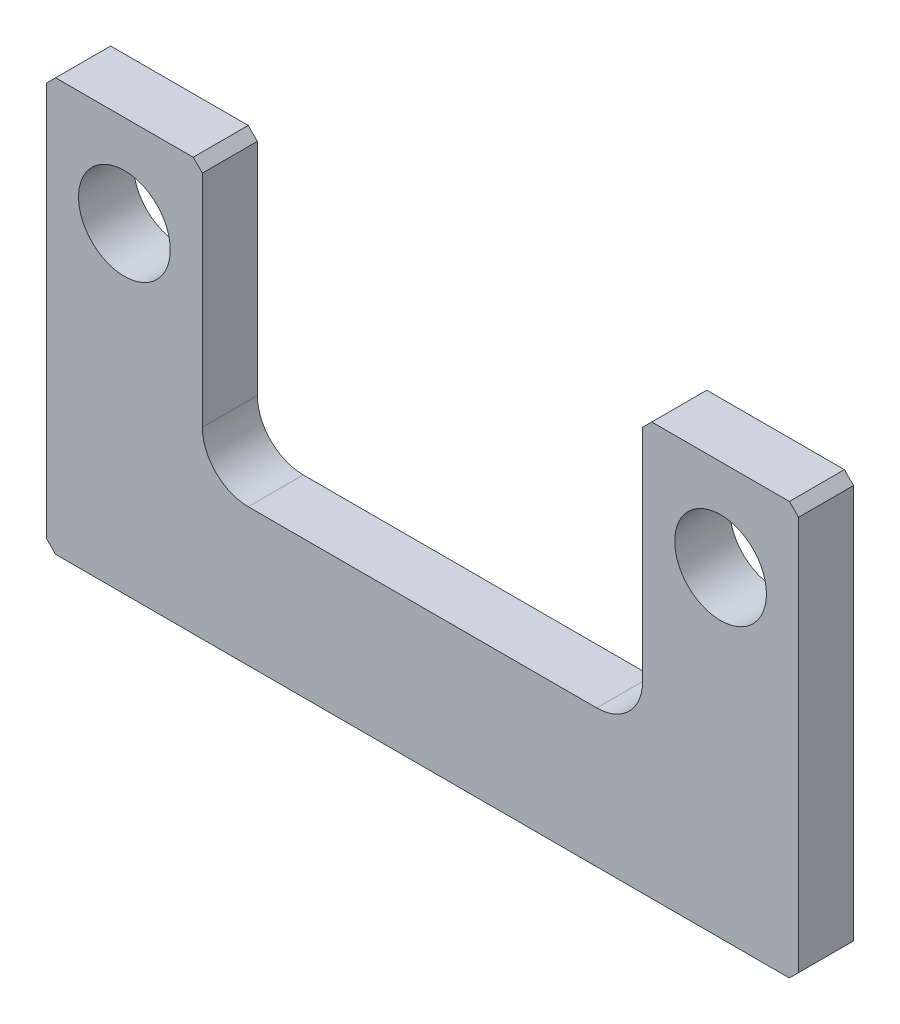
SolidWorks part; units mm, degrees
ref_plane "前视基准面" through (0, 0, 0) normal (0, 0, 1) x (1, 0, 0)
ref_plane "上视基准面" through (0, 0, 0) normal (0, 1, 0) x (1, 0, 0)
ref_plane "右视基准面" through (0, 0, 0) normal (1, 0, 0) x (0, 0, -1)
sketch "草图1" plane through (0, 0, 0) normal (0, 0, 1) x (1, 0, 0)
  line L0 (-82, -70) -> (-82, 20)
  line L1 (-82, 20) -> (-48, 20)
  line L2 (-48, 20) -> (-48, -40)
  line L3 (-48, -40) -> (48, -40)
  line L4 (48, -40) -> (48, 20)
  line L5 (48, 20) -> (82, 20)
  line L6 (82, 20) -> (82, -70)
  line L7 (82, -70) -> (-82, -70)
  circle A0 centre (-65, 0) radius 10
  circle A1 centre (65, 0) radius 10
extrude "凸台-拉伸1" add sketch "草图1" along normal mid plane 12
fillet "圆角1" radius 10 2 edges at (48, -40, 0) (-48, -40, 0)
chamfer "倒角1" distance 2 angle 45 6 edges at (82, -70, 0) (-82, -70, 0) (82, 20, 0) (48, 20, 0) (-48, 20, 0) (-82, 20, 0)
equation "\"D3@草图1\"=\"D2@草图1\""
equation "\"D6@草图1\"=\"D4@草图1\""
equation "\"D8@草图1\"=\"D7@草图1\""
